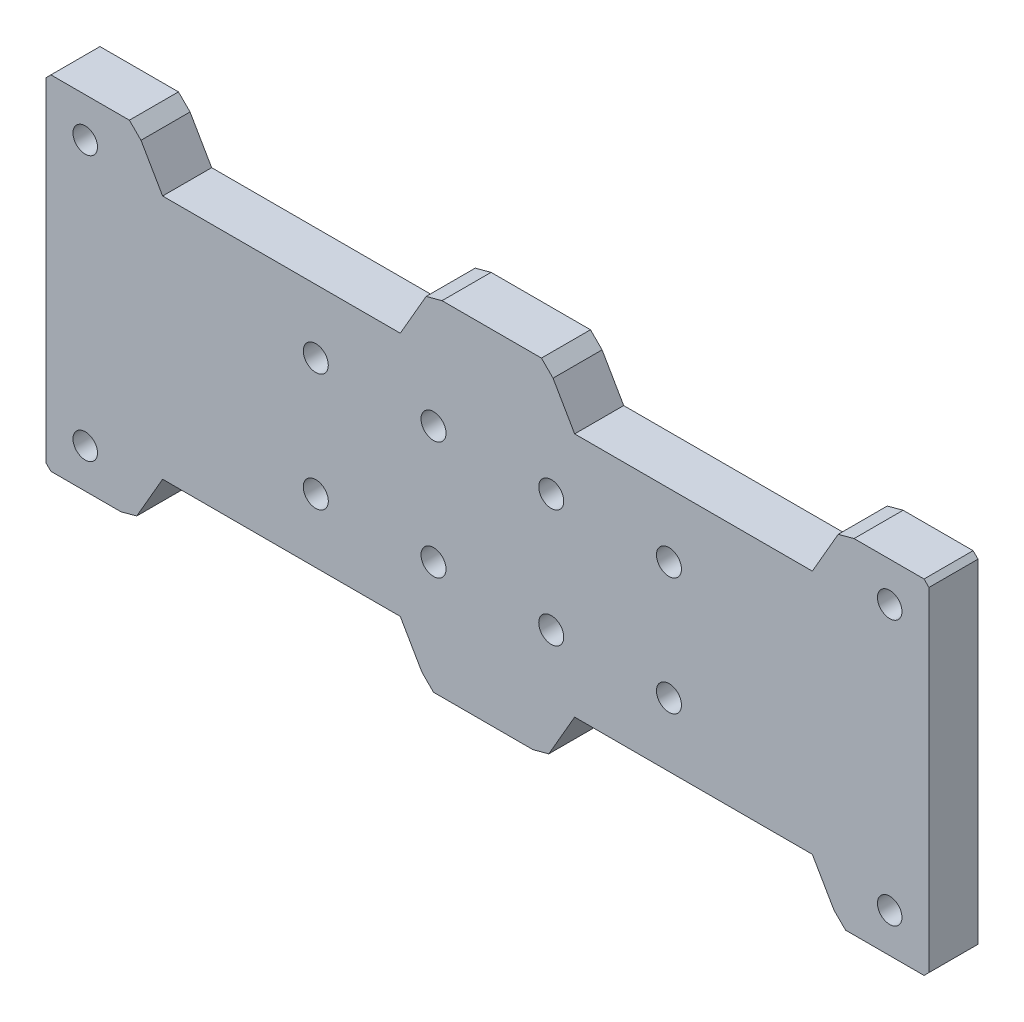
from build123d import *
from OCP.BRepFilletAPI import BRepFilletAPI_MakeChamfer

# Parameters (mm, degrees)
SKETCH1_W           = 180
SKETCH1_H           = 70
BOSS_EXTRUDE1_DEPTH = 10
CUT_EXTRUDE1_DEPTH  = 98.082439195
SKETCH3_R           = 2.5
CUT_EXTRUDE2_DEPTH  = 98.082439195
CHAMFER1_SIZE       = 1
CHAMFER1_SIZE2      = 2.732050808
SKETCH4_R           = 2.55
CUT_EXTRUDE3_DEPTH  = 98.082439195


with BuildPart() as part:
    # Sketch1 → Boss-Extrude1 (new body)
    with BuildSketch(Plane.XY):
        Rectangle(SKETCH1_W, SKETCH1_H)
    extrude(amount=BOSS_EXTRUDE1_DEPTH)

    # Sketch2 → Cut-Extrude1 (cut, through all)
    with BuildSketch(Plane.XY.offset(10)):
        Polygon((-72, 35), (-66.226497308, 25), (-17.773502692, 25), (-12, 35), align=None)
        Polygon((72, 35), (12, 35), (17.773502692, 25), (66.226497308, 25), align=None)
        Polygon((72, -35), (66.226497308, -25), (17.773502692, -25), (12, -35), align=None)
        Polygon((-72, -35), (-12, -35), (-17.773502692, -25), (-66.226497308, -25), align=None)
    extrude(amount=-CUT_EXTRUDE1_DEPTH, mode=Mode.SUBTRACT)

    # Sketch3 → Cut-Extrude2 (cut, through all)
    with BuildSketch(Plane.XY.offset(10)):
        with Locations((-82, 27)):
            Circle(SKETCH3_R)
        with Locations(Location((82, 27, 0), (0, 0, 180))):
            Circle(SKETCH3_R)
        with Locations((82, -27)):
            Circle(SKETCH3_R)
        with Locations(Location((-82, -27, 0), (0, 0, 180))):
            Circle(SKETCH3_R)
    extrude(amount=-CUT_EXTRUDE2_DEPTH, mode=Mode.SUBTRACT)

    # Chamfer1: one chamfer whose edges measure the first distance from different faces: ONE call of the kernel's chamfer builder (chamfer() names one face for all edges)
    chamfer1_edges_1 = [part.edges().sort_by_distance(p)[0] for p in [
        (-72, -35, 5),
    ]]
    chamfer1_side_1 = [part.faces().sort_by_distance(p)[0] for p in [
        (-69.113248654, -30, 5),
    ]]
    chamfer1_edges_2 = [part.edges().sort_by_distance(p)[0] for p in [
        (-12, -35, 5),
    ]]
    chamfer1_side_2 = [part.faces().sort_by_distance(p)[0] for p in [
        (0, -35, 5),
    ]]
    chamfer1_edges_3 = [part.edges().sort_by_distance(p)[0] for p in [
        (72, -35, 5),
    ]]
    chamfer1_side_3 = [part.faces().sort_by_distance(p)[0] for p in [
        (81, -35, 5),
    ]]
    chamfer1_edges_4 = [part.edges().sort_by_distance(p)[0] for p in [
        (12, -35, 5),
    ]]
    chamfer1_side_4 = [part.faces().sort_by_distance(p)[0] for p in [
        (14.886751346, -30, 5),
    ]]
    chamfer1_edges_5 = [part.edges().sort_by_distance(p)[0] for p in [
        (72, 35, 5),
    ]]
    chamfer1_side_5 = [part.faces().sort_by_distance(p)[0] for p in [
        (69.113248654, 30, 5),
    ]]
    chamfer1_edges_6 = [part.edges().sort_by_distance(p)[0] for p in [
        (12, 35, 5),
    ]]
    chamfer1_side_6 = [part.faces().sort_by_distance(p)[0] for p in [
        (0, 35, 5),
    ]]
    chamfer1_edges_7 = [part.edges().sort_by_distance(p)[0] for p in [
        (-72, 35, 5),
    ]]
    chamfer1_side_7 = [part.faces().sort_by_distance(p)[0] for p in [
        (-81, 35, 5),
    ]]
    chamfer1_edges_8 = [part.edges().sort_by_distance(p)[0] for p in [
        (-12, 35, 5),
    ]]
    chamfer1_side_8 = [part.faces().sort_by_distance(p)[0] for p in [
        (-14.886751346, 30, 5),
    ]]
    chamfer1_edges_9 = [part.edges().sort_by_distance(p)[0] for p in [
        (90, -35, 5),
        (-90, -35, 5),
        (-90, 35, 5),
        (90, 35, 5),
    ]]
    chamfer1 = BRepFilletAPI_MakeChamfer(part.part.solid().wrapped)
    for e in chamfer1_edges_1:
        chamfer1.Add(CHAMFER1_SIZE, CHAMFER1_SIZE2, e.wrapped, chamfer1_side_1[0].wrapped)  # the first distance lies on this face
    for e in chamfer1_edges_2:
        chamfer1.Add(CHAMFER1_SIZE, CHAMFER1_SIZE2, e.wrapped, chamfer1_side_2[0].wrapped)  # the first distance lies on this face
    for e in chamfer1_edges_3:
        chamfer1.Add(CHAMFER1_SIZE, CHAMFER1_SIZE2, e.wrapped, chamfer1_side_3[0].wrapped)  # the first distance lies on this face
    for e in chamfer1_edges_4:
        chamfer1.Add(CHAMFER1_SIZE, CHAMFER1_SIZE2, e.wrapped, chamfer1_side_4[0].wrapped)  # the first distance lies on this face
    for e in chamfer1_edges_5:
        chamfer1.Add(CHAMFER1_SIZE, CHAMFER1_SIZE2, e.wrapped, chamfer1_side_5[0].wrapped)  # the first distance lies on this face
    for e in chamfer1_edges_6:
        chamfer1.Add(CHAMFER1_SIZE, CHAMFER1_SIZE2, e.wrapped, chamfer1_side_6[0].wrapped)  # the first distance lies on this face
    for e in chamfer1_edges_7:
        chamfer1.Add(CHAMFER1_SIZE, CHAMFER1_SIZE2, e.wrapped, chamfer1_side_7[0].wrapped)  # the first distance lies on this face
    for e in chamfer1_edges_8:
        chamfer1.Add(CHAMFER1_SIZE, CHAMFER1_SIZE2, e.wrapped, chamfer1_side_8[0].wrapped)  # the first distance lies on this face
    for e in chamfer1_edges_9:
        chamfer1.Add(CHAMFER1_SIZE, e.wrapped)
    add(Compound.cast(chamfer1.Shape()), mode=Mode.REPLACE)

    # Sketch4 → Cut-Extrude3 (cut, through all)
    with BuildSketch(Plane.XY.offset(10)):
        with Locations((-35, 12)):
            Circle(SKETCH4_R)
        with Locations((-11, 12)):
            Circle(SKETCH4_R)
        with Locations((13, 12)):
            Circle(SKETCH4_R)
        with Locations((37, 12)):
            Circle(SKETCH4_R)
        with Locations(Location((37, -12, 0), (0, 0, 180))):
            Circle(SKETCH4_R)
        with Locations(Location((13, -12, 0), (0, 0, 180))):
            Circle(SKETCH4_R)
        with Locations(Location((-11, -12, 0), (0, 0, 180))):
            Circle(SKETCH4_R)
        with Locations(Location((-35, -12, 0), (0, 0, 180))):
            Circle(SKETCH4_R)
    extrude(amount=-CUT_EXTRUDE3_DEPTH, mode=Mode.SUBTRACT)


solid = part.part
